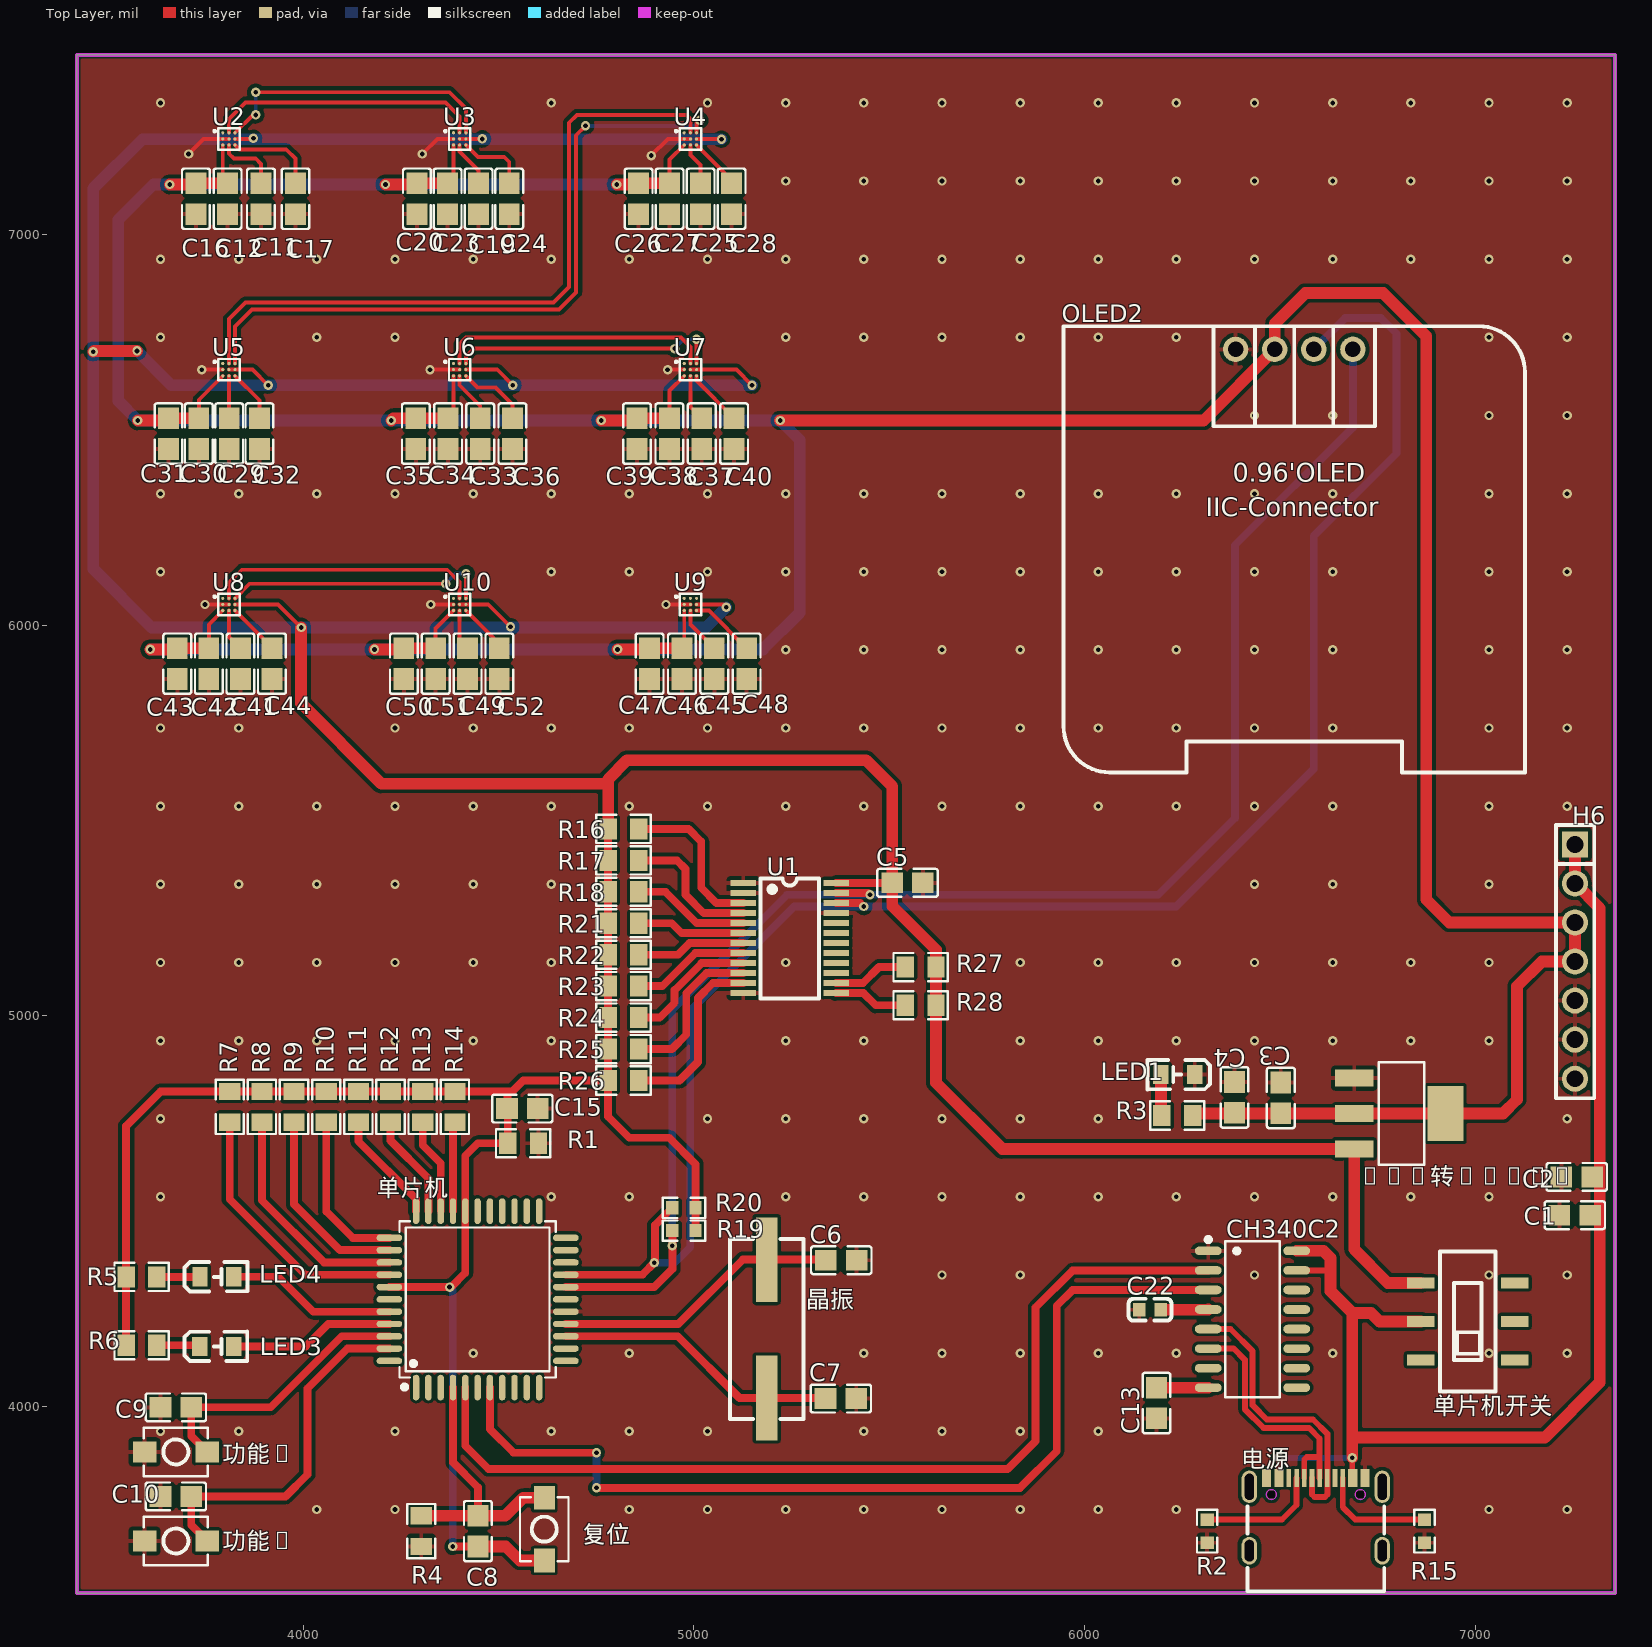
[diagram p0: Top Layer view]
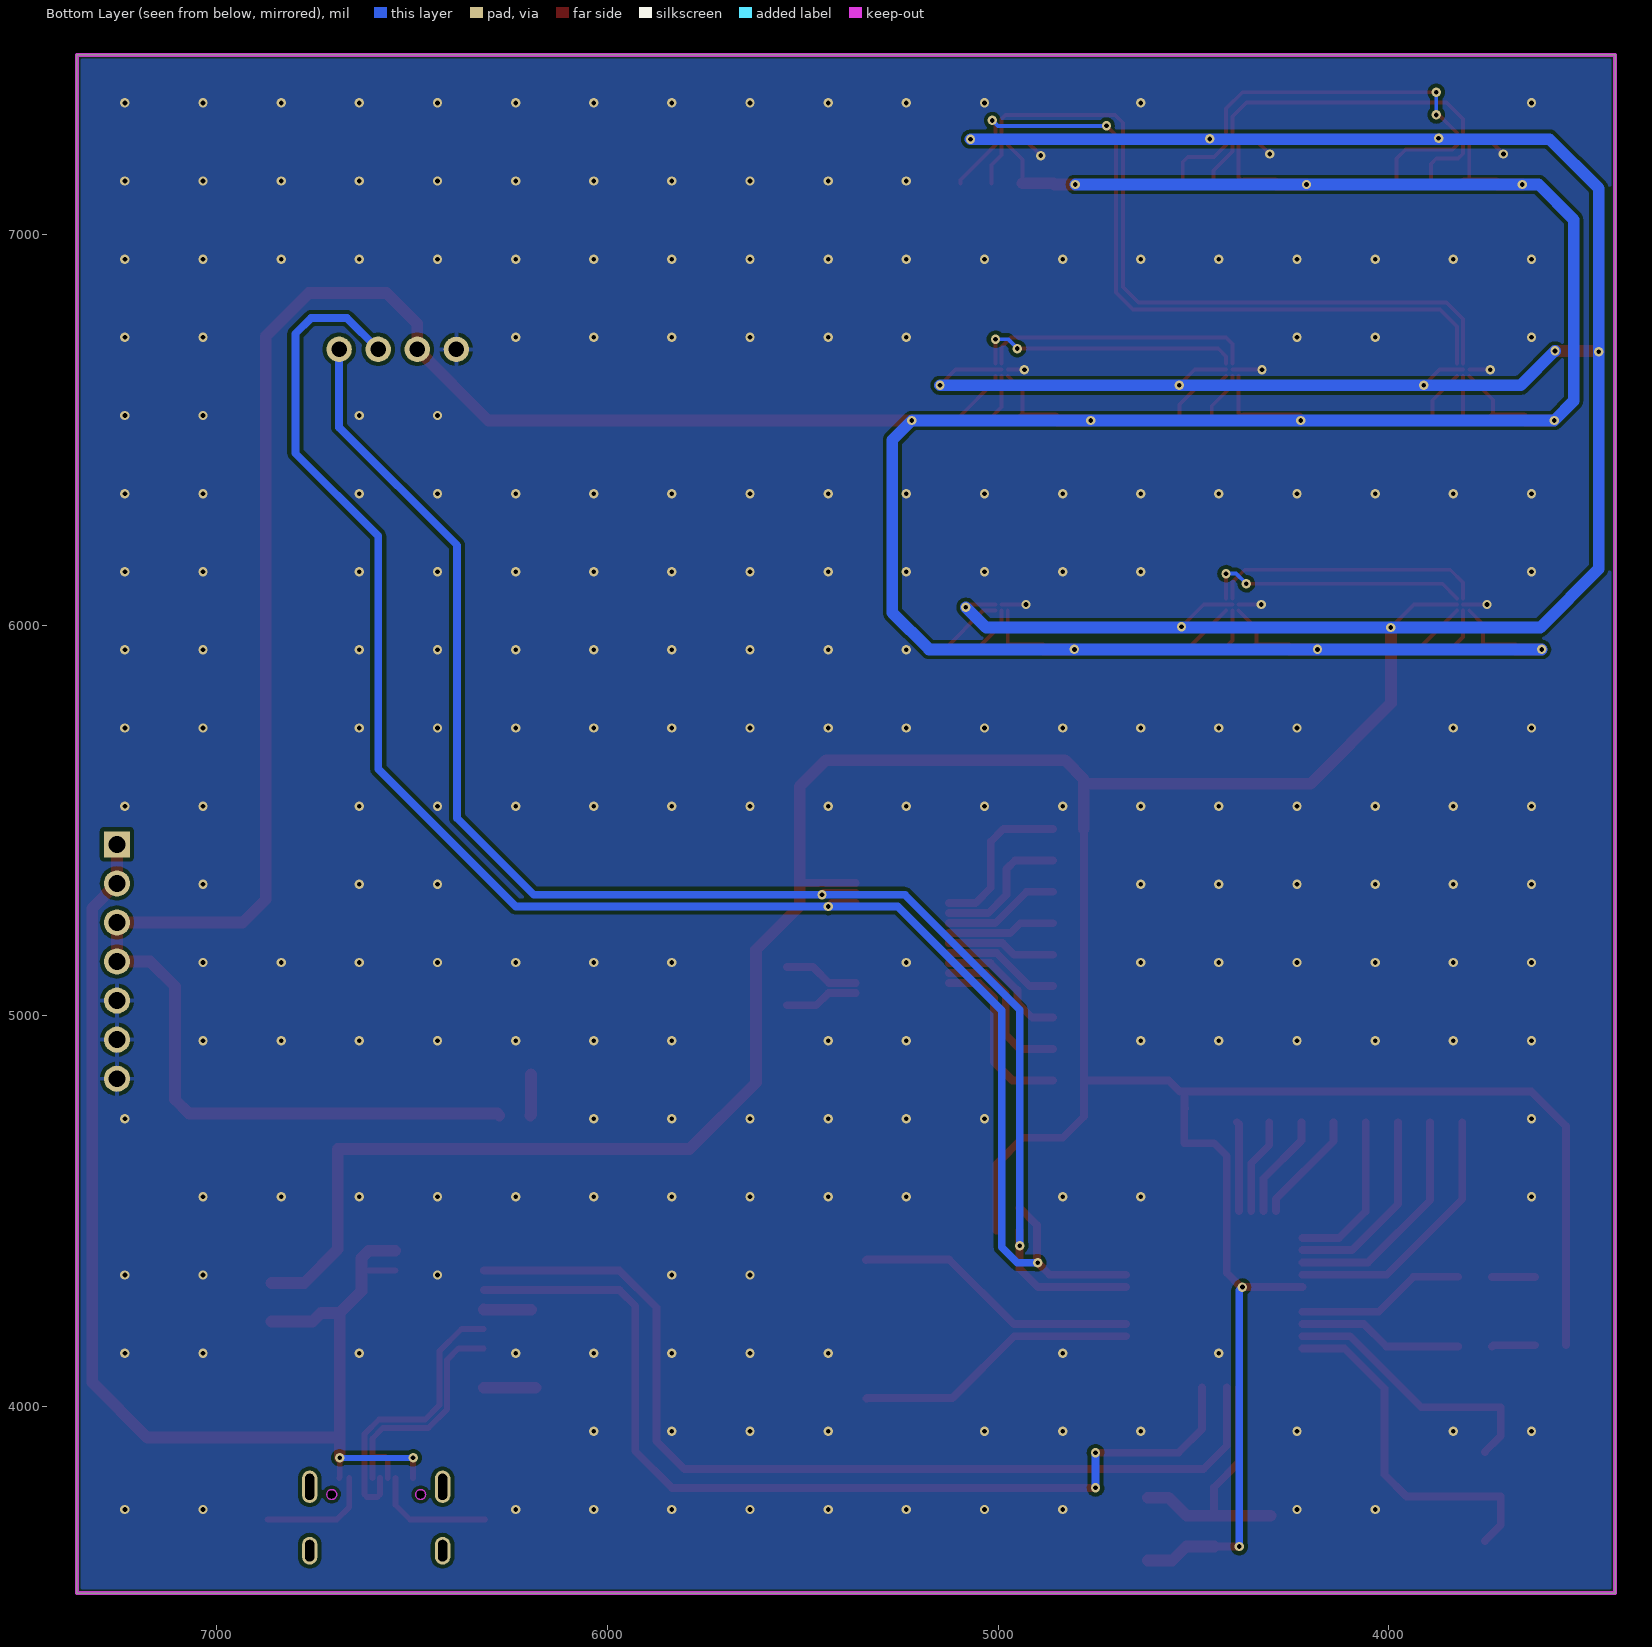
[diagram p1: Bottom Layer view, seen from below]
# Altium PCB MISC75115.pcbdoc
Units mil, origin at the board's own origin, x right, y up, seen from the top; angles counter-clockwise.
Board outline 3937.01 x 3937.01 mil, 2 copper layers (Top Layer, Bottom Layer), stack 62.206 mil thick; 101 components, 93 nets, 370 pads, 280 vias.

## Layer stack, top to bottom
Top Solder Mask Layer: solder mask 0.394, Dk 3.3
Top Layer: signal copper 1.379
Dielectric1: surface 59.449, FR4, Dk 4.5
Bottom Layer: signal copper 1.378
Bottom Solder Mask Layer: solder mask 0.394, Dk 3.3

## Board outline
3420.99,7459.65 3420.99,3522.65 7358,3522.65 7358,7459.65

## Design rules (kind name [scope] priority, off if disabled: settings)
BoardOutlineClearance copperThickness2oz_1 [All] p2 off: genericclearance=7.99 ignorepadtopadclearanceinfootprint=FALSE except(0: Arc-SplitContinuation Track-SplitContinuation SMDPad-SplitContinuation THPad-SplitContinuation Via-SplitContinuation Fill-SplitContinuation Region-SplitContinuation Poly-SplitContinuation Text-SplitContinuation Hole-SplitContinuation; 5.98: Arc-CutoutEdge SMDPad-CutoutEdge THPad-CutoutEdge Via-CutoutEdge Fill-CutoutEdge Region-CutoutEdge Text-CutoutEdge; 6.93: Hole-OutlineEdge Hole-CutoutEdge; 10: Poly-OutlineEdge Poly-CutoutEdge; 11.81: Arc-OutlineEdge Track-OutlineEdge SMDPad-OutlineEdge THPad-OutlineEdge Via-OutlineEdge Fill-OutlineEdge Region-OutlineEdge Text-OutlineEdge Track-CutoutEdge)
BoardOutlineClearance Plane_innerPlane_1 [All] p4 off: genericclearance=4.02 ignorepadtopadclearanceinfootprint=FALSE except(0: Arc-SplitContinuation Track-SplitContinuation SMDPad-SplitContinuation THPad-SplitContinuation Via-SplitContinuation Fill-SplitContinuation Region-SplitContinuation Poly-SplitContinuation Text-SplitContinuation Hole-SplitContinuation; 6: SMDPad-CutoutEdge THPad-CutoutEdge Via-CutoutEdge Fill-CutoutEdge Region-CutoutEdge Text-CutoutEdge; 6.93: Hole-OutlineEdge Hole-CutoutEdge; 10: Poly-OutlineEdge Poly-CutoutEdge; 11.8: Arc-OutlineEdge Track-OutlineEdge SMDPad-OutlineEdge THPad-OutlineEdge Via-OutlineEdge Fill-OutlineEdge Region-OutlineEdge Text-OutlineEdge; 11.81: Arc-CutoutEdge Track-CutoutEdge)
BoardOutlineClearance Copper_copperRegion_1 [All] p6 off: genericclearance=4.02 ignorepadtopadclearanceinfootprint=FALSE except(0: Arc-SplitContinuation Track-SplitContinuation SMDPad-SplitContinuation THPad-SplitContinuation Via-SplitContinuation Fill-SplitContinuation Region-SplitContinuation Poly-SplitContinuation Text-SplitContinuation Hole-SplitContinuation; 6: SMDPad-CutoutEdge THPad-CutoutEdge Via-CutoutEdge Fill-CutoutEdge Region-CutoutEdge Text-CutoutEdge; 6.93: Hole-OutlineEdge Hole-CutoutEdge; 10: Poly-OutlineEdge Poly-CutoutEdge; 11.8: Arc-OutlineEdge Track-OutlineEdge SMDPad-OutlineEdge THPad-OutlineEdge Via-OutlineEdge Fill-OutlineEdge Region-OutlineEdge Text-OutlineEdge; 11.81: Arc-CutoutEdge Track-CutoutEdge)
BoardOutlineClearance copperThickness1oz_1 [All] p8: genericclearance=4.02 ignorepadtopadclearanceinfootprint=FALSE except(0: Arc-SplitContinuation Track-SplitContinuation SMDPad-SplitContinuation THPad-SplitContinuation Via-SplitContinuation Fill-SplitContinuation Region-SplitContinuation Poly-SplitContinuation Text-SplitContinuation Hole-SplitContinuation; 6: SMDPad-CutoutEdge THPad-CutoutEdge Via-CutoutEdge Fill-CutoutEdge Region-CutoutEdge Text-CutoutEdge; 6.93: Hole-OutlineEdge Hole-CutoutEdge; 10: Poly-OutlineEdge Poly-CutoutEdge; 11.8: Arc-OutlineEdge Track-OutlineEdge SMDPad-OutlineEdge THPad-OutlineEdge Via-OutlineEdge Fill-OutlineEdge Region-OutlineEdge Text-OutlineEdge; 11.81: Arc-CutoutEdge Track-CutoutEdge)
Clearance copperThickness2oz [All] p1 off: gap=7.99 ignorepadtopadclearanceinfootprint=FALSE except(5.98: SMDPad-Track SMDPad-SMDPad THPad-Track SMDPad-THPad THPad-THPad Track-Via SMDPad-Via THPad-Via Via-Via Fill-Track Region-Track Fill-SMDPad Region-SMDPad Fill-THPad Region-THPad Fill-Via Region-Via Fill-Fill Fill-Region Region-Region Arc-Track Arc-SMDPad Arc-THPad Arc-Via Fill-Arc Region-Arc Arc-Arc Text-Track SMDPad-Text Text-THPad Text-Via Fill-Text Region-Text Arc-Text Text-Text; 6.93: Hole-Track Hole-SMDPad Hole-THPad Hole-Via Fill-Hole Region-Hole Hole-Arc Hole-Text; 10: Poly-Track Poly-SMDPad Poly-THPad Poly-Via Poly-Fill Poly-Region Poly-Poly Poly-Arc Poly-Text Poly-Hole)
Clearance Plane_innerPlane [All] p3 off: gap=4.02 ignorepadtopadclearanceinfootprint=FALSE except(4.33: SMDPad-Track SMDPad-SMDPad SMDPad-THPad; 5.98: THPad-Track THPad-THPad Track-Via SMDPad-Via THPad-Via Via-Via Fill-Track Region-Track Fill-SMDPad Region-SMDPad Fill-THPad Region-THPad Fill-Via Region-Via Fill-Fill Fill-Region Region-Region; 6: Arc-Track Arc-SMDPad Arc-THPad Arc-Via Fill-Arc Region-Arc Arc-Arc Text-Track SMDPad-Text Text-THPad Text-Via Fill-Text Region-Text Arc-Text Text-Text; 6.93: Hole-Track Hole-SMDPad Hole-THPad Hole-Via Fill-Hole Region-Hole Hole-Arc Hole-Text; 10: Poly-Track Poly-SMDPad Poly-THPad Poly-Via Poly-Fill Poly-Region Poly-Poly Poly-Arc Poly-Text Poly-Hole)
Clearance Copper_copperRegion [All] p5 off: gap=4.02 ignorepadtopadclearanceinfootprint=FALSE except(4.33: SMDPad-Track SMDPad-SMDPad SMDPad-THPad; 5.98: THPad-Track THPad-THPad Track-Via SMDPad-Via THPad-Via Via-Via Fill-Track Region-Track Fill-SMDPad Region-SMDPad Fill-THPad Region-THPad Fill-Via Region-Via Fill-Fill Fill-Region Region-Region; 6: Arc-Track Arc-SMDPad Arc-THPad Arc-Via Fill-Arc Region-Arc Arc-Arc Text-Track SMDPad-Text Text-THPad Text-Via Fill-Text Region-Text Arc-Text Text-Text; 6.93: Hole-Track Hole-SMDPad Hole-THPad Hole-Via Fill-Hole Region-Hole Hole-Arc Hole-Text; 10: Poly-Track Poly-SMDPad Poly-THPad Poly-Via Poly-Fill Poly-Region Poly-Poly Poly-Arc Poly-Text Poly-Hole)
Clearance copperThickness1oz [All] p7: gap=4.02 ignorepadtopadclearanceinfootprint=FALSE except(4.33: SMDPad-Track SMDPad-SMDPad SMDPad-THPad; 5.98: THPad-Track THPad-THPad Track-Via SMDPad-Via THPad-Via Via-Via Fill-Track Region-Track Fill-SMDPad Region-SMDPad Fill-THPad Region-THPad Fill-Via Region-Via Fill-Fill Fill-Region Region-Region; 6: Arc-Track Arc-SMDPad Arc-THPad Arc-Via Fill-Arc Region-Arc Arc-Arc Text-Track SMDPad-Text Text-THPad Text-Via Fill-Text Region-Text Arc-Text Text-Text; 6.93: Hole-Track Hole-SMDPad Hole-THPad Hole-Via Fill-Hole Region-Hole Hole-Arc Hole-Text; 7.87: Poly-SMDPad; 10: Poly-Track Poly-THPad Poly-Via Poly-Fill Poly-Region Poly-Poly Poly-Arc Poly-Text Poly-Hole)
DiffPairsRouting differentialPair [All] p1: maxlimit=6 minlimit=6 mostfreqgap=6 toplayer_minwidth=5 toplayer_prefwidth=10 toplayer_maxwidth=100 toplayer_mingap=6 toplayer_prefgap=6 toplayer_maxgap=6 bottomlayer_minwidth=5 bottomlayer_prefwidth=10 bottomlayer_maxwidth=100 bottomlayer_mingap=6 bottomlayer_prefgap=6 bottomlayer_maxgap=6 maxuncoupledlength=10
HoleToHoleClearance otherClearance [All] p1: gap=11.81 allowstackedmicrovias=TRUE
Length netLength [All] p1: minlimit=0 maxlimit=0
MatchedLengths netLengthTolerance [All] p1: tolerance=1000
PasteMaskExpansion pasteMaskExpansion [All] p1: expansion=0
PlaneConnect innerPlane [All] p1: planeconnectstyle=Relief reliefexpansion=20 reliefentries=4 reliefconductorwidth=10 reliefairgap=10
PolygonConnect copperRegion [(InNet('GND'))] p1: connectstyle=Relief reliefconductorwidth=10 reliefentries=4 polygonreliefangle="90 Angle" airgapwidth=10 via.connectstyle=Relief via.reliefconductorwidth=10 via.reliefentries=4 via.polygonreliefangle="90 Angle" via.airgapwidth=10
RoutingVias viaSize [All] p1: holewidth=12.01 width=24.02 viastyle="Through Hole" minholewidth=11.81 minwidth=19.68 maxholewidth=248.03 maxwidth=393.7
SolderMaskExpansion solderMaskExpansion [IsVia] p1: expansion=-1000 istentingtop=TRUE
SolderMaskExpansion solderMaskExpansion [All] p2: expansion=2 istentingtop=FALSE
Width copperThickness2oz_2 [All] p1 off: maxlimit=100 minlimit=8 preferedwidth=10
Width copperThickness1oz_2 [All] p2: maxlimit=100 minlimit=5 preferedwidth=10

## Components (designator, comment, footprint, x,y, rotation, side; value= is the part's Value field where it differs from the comment)
+5v转+3.3v "AMS1117-3.3" SOT-223-3_L6.5-W3.4-P2.30-LS7.0-BR 6807.33,4750.06 r180 top (schematic designator +5vת+3.3v)
C1 "10UF" C0805 7254.78,4489.81 r0 top
C2 "100nF" C0805 7259.73,4587.87 r0 top
C3 "100nF" C0805 6502.33,4790.06 r270 top
C4 "10UF" C0805 6383.84,4791.38 r270 top
C5 "100nF" C0805 5546.9,5340.64 r0 top
C6 "22PF" C0805 5377.38,4374.53 r0 top
C7 "22PF" C0805 5376.25,4020.68 r0 top
C8 "10UF" C0805 4447.29,3681.27 r90 top
C9 "0.1uf" C0805 3674.24,3998.11 r0 top
C10 "0.1uf" C0805 3674.24,3770.08 r0 top
C11 "2.2uF" C0805 3892.09,7091.39 r270 top
C12 "10UF" C0805 3806.59,7091.39 r270 top
C13 "0.1UF" C0805 6184.26,4009.17 r90 top
C15 "0.1uF" C0805 4561.03,4762.76 r180 top
C16 "0.1UF" C0805 3725.76,7091.39 r90 top
C17 "0.1UF" C0805 3980.5,7091.39 r90 top
C19 "2.2uF" C0805 4449.23,7091.39 r270 top
C20 "10UF" C0805 4291.41,7091.39 r270 top
C22 "100nF" C0603 6167.65,4248 r0 top
C23 "0.1UF" C0805 4369.72,7091.39 r90 top
C24 "0.1UF" C0805 4527.68,7091.39 r90 top
C25 "2.2uF" C0805 5017.41,7091.39 r270 top
C26 "10UF" C0805 4858.71,7091.39 r270 top
C27 "0.1UF" C0805 4938.06,7091.39 r90 top
C28 "0.1UF" C0805 5096.75,7091.39 r90 top
C29 "2.2uF" C0805 3810.7,6490.3 r270 top
C30 "10UF" C0805 3733.09,6490.3 r270 top
C31 "0.1UF" C0805 3655.48,6490.3 r90 top
C32 "0.1UF" C0805 3888.3,6490.3 r90 top
C33 "2.2uF" C0805 4453.38,6490.3 r270 top
C34 "10UF" C0805 4370.98,6490.3 r270 top
C35 "0.1UF" C0805 4288.57,6490.3 r90 top
C36 "0.1UF" C0805 4535.78,6490.3 r90 top
C37 "2.2uF" C0805 5020.24,6490.3 r270 top
C38 "10UF" C0805 4937.42,6490.3 r270 top
C39 "0.1UF" C0805 4854.6,6490.3 r90 top
C40 "0.1UF" C0805 5103.06,6490.3 r90 top
C41 "2.2uF" C0805 3839.49,5901.41 r270 top
C42 "10UF" C0805 3758.74,5901.41 r270 top
C43 "0.1UF" C0805 3677.99,5901.41 r90 top
C44 "0.1UF" C0805 3920.25,5901.41 r90 top
C45 "2.2uF" C0805 5052.43,5901.41 r270 top
C46 "10UF" C0805 4969.58,5901.41 r270 top
C47 "0.1UF" C0805 4886.73,5901.41 r90 top
C48 "0.1UF" C0805 5135.28,5901.41 r90 top
C49 "2.2uF" C0805 4420.81,5901.41 r270 top
C50 "10UF" C0805 4257.85,5901.41 r270 top
C51 "0.1UF" C0805 4339.33,5901.41 r90 top
C52 "0.1UF" C0805 4502.28,5901.41 r90 top
CH340C2 "CH340C" SOP-16_L10.0-W3.9-P1.27-LS6.0-BL 6429.8,4223.56 r270 top
H6 "" HDR-TH_7P-P2.54-V-M 7255.44,5139.1 r270 top
LED1 "" LED_0805 6236.85,4849.96 r180 top
LED3 "" LED_0805 3781.01,4153.88 r0 top
LED4 "" LED_0805 3781.45,4331.99 r0 top
OLED2 "0.96OLED_4P_MODULE_JX" 0.96OLED_4P 6536.78,6705.99 r0 top
R1 "1K" R0805 4563.04,4674.02 r180 top
R2 "5.1K" R0603 6313.91,3681.25 r90 top
R3 "1K" R0805 6237.33,4745.06 r180 top
R4 "10K" R0805 4302.29,3681.27 r90 top
R5 "1K" R0805 3586.45,4331.99 r180 top
R6 "1K" R0805 3586.45,4156.99 r180 top
R7 "10K" R0805 3812.09,4767.13 r90 top
R8 "10K" R0805 3894.42,4767.13 r90 top
R9 "10K" R0805 3976.74,4767.13 r90 top
R10 "10K" R0805 4059.06,4767.13 r90 top
R11 "10K" R0805 4141.39,4767.13 r90 top
R12 "10K" R0805 4223.71,4767.13 r90 top
R13 "10K" R0805 4306.03,4767.13 r90 top
R14 "10K" R0805 4388.35,4767.13 r90 top
R15 "5.1K" R0603 6870.09,3681.25 r90 top
R16 "10K" R0805 4820.05,5478.59 r0 top
R17 "4.7K" R0805 4820.05,5398.1 r0 top
R18 "4.7K" R0805 4820.05,5317.6 r0 top
R19 "4.7K" R0603 4974.74,4450.48 r180 top
R20 "4.7K" R0603 4974.74,4508.71 r180 top
R21 "4.7K" R0805 4820.05,5237.11 r0 top
R22 "4.7K" R0805 4820.05,5156.62 r0 top
R23 "4.7K" R0805 4820.05,5076.13 r0 top
R24 "4.7K" R0805 4820.05,4995.64 r0 top
R25 "4.7K" R0805 4820.05,4915.15 r0 top
R26 "4.7K" R0805 4820.05,4834.65 r0 top
R27 "4.7K" R0805 5580.44,5125 r0 top
R28 "4.7K" R0805 5580.44,5027.11 r0 top
U1 "TCA9548APWR" TSSOP-24_L7.8-W4.4-P0.65-LS6.4-BL 5245.63,5199.05 r270 top
U2 "BMM350" WLCSP-9_L1.3-W1.3-R3-C3-P0.40-TL 3810.08,7244.57 r0 top
U3 "BMM350" WLCSP-9_L1.3-W1.3-R3-C3-P0.40-TL 4400.64,7244.57 r0 top
U4 "BMM350" WLCSP-9_L1.3-W1.3-R3-C3-P0.40-TL 4991.21,7244.57 r0 top
U5 "BMM350" WLCSP-9_L1.3-W1.3-R3-C3-P0.40-TL 3810.08,6654.02 r0 top
U6 "BMM350" WLCSP-9_L1.3-W1.3-R3-C3-P0.40-TL 4400.64,6654.02 r0 top
U7 "BMM350" WLCSP-9_L1.3-W1.3-R3-C3-P0.40-TL 4991.21,6654.02 r0 top
U8 "BMM350" WLCSP-9_L1.3-W1.3-R3-C3-P0.40-TL 3810.08,6053.06 r0 top
U9 "BMM350" WLCSP-9_L1.3-W1.3-R3-C3-P0.40-TL 4991.21,6053.06 r0 top
U10 "BMM350" WLCSP-9_L1.3-W1.3-R3-C3-P0.40-TL 4400.64,6053.06 r0 top
功能1 "Tact switch 3*4*H" SW-SMD_L4.0-W2.9-LS5.0 3674.24,3884.1 r180 top
功能2 "Tact switch 3*4*H" SW-SMD_L4.0-W2.9-LS5.0 3674.24,3656.07 r180 top
单片机 "STC89C52RC-40I-LQFP44" LQFP-44_L10.0-W10.0-P0.80-LS12.0-BL 4446.58,4274.46 r0 top
单片机开关 "SS-3235S-L1" SW-SMD_SS-3235S-LX 6980.85,4217.96 r270 top
复位 "Tact switch 3*4*H" SW-SMD_L4.0-W2.9-LS5.0 4617.29,3686.27 r270 top
晶振 "12MHz" CRYSTAL-SMD_L11.4-W4.7-LS12.7 5186.58,4199.09 r270 top
电源 "Type-C" USB-C-SMD_TYPE-C16PIN 6592,3724.3 r0 top

## Footprints (in the part's own frame and the unit in brackets; to place one, negate y for a bottom-side part, rotate by r counter-clockwise, add the part's x,y. Pads: shape width x height; smd on the part's side, far side on the other; paste and mask are expansions set on the pad)
0.96OLED_4P [mm]
  round 1.65 hole 1 copper offset 0,0: 1(-3.81,-0.001) 2(-1.27,0.002) 3(1.27,0.002) 4(3.81,0.002)
  silkscreen extent -15,-27.5 15,1.5
C0603 [mm]
  rect 0.8x0.9 smd: 1(-0.7,0) 2(0.7,0)
  silkscreen extent -1.39,-0.71 1.39,0.71
C0805 [mm]
  rect 1.41x1.35 smd paste-100 mask+0.051: 1(-1,0) 2(1,0)
  silkscreen extent -1.96,-0.9 1.96,0.9
CRYSTAL-SMD_L11.4-W4.7-LS12.7 [mm]
  rect 5.5x1.4 smd: 1(-4.5,0) 2(4.5,0)
  silkscreen extent -5.85,-2.4 5.85,2.4
HDR-TH_7P-P2.54-V-M [mm]
  rect 1.7x1.7 hole 1.1: 1(-7.62,0)
  round 1.7 hole 1.1: 2(-5.08,0) 3(-2.54,0) 4(0,0) 5(2.54,0) 6(5.08,0) 7(7.62,0)
  silkscreen extent -8.89,-1.25 8.89,1.25
LED_0805 [mm]
  rect 1x1.25 smd paste+0 mask+0.051: 1(-1.15,0.005) 2(1.05,0.005)
  silkscreen extent -2.15,-0.94 1.93,0.97
LQFP-44_L10.0-W10.0-P0.80-LS12.0-BL [mm]
  oval 0.42x1.67 smd: 1(-4,-5.735) 2(-3.2,-5.735) 3(-2.4,-5.735) 4(-1.6,-5.735) 5(-0.8,-5.735) 6(0,-5.735) 7(0.8,-5.735) 8(1.6,-5.735) 9(2.4,-5.735) 10(3.2,-5.735) 11(4,-5.735) 23(4,5.735) 24(3.2,5.735) 25(2.4,5.735) 26(1.6,5.735) 27(0.8,5.735) 28(0,5.735) 29(-0.8,5.735) 30(-1.6,5.735) 31(-2.4,5.735) 32(-3.2,5.735) 33(-4,5.735)
  oval 1.67x0.42 smd: 12(5.735,-4) 13(5.735,-3.2) 14(5.735,-2.4) 15(5.735,-1.6) 16(5.735,-0.8) 17(5.735,0) 18(5.735,0.8) 19(5.735,1.6) 20(5.735,2.4) 21(5.735,3.2) 22(5.735,4) 34(-5.735,4) 35(-5.735,3.2) 36(-5.735,2.4) 37(-5.735,1.6) 38(-5.735,0.8) 39(-5.735,0) 40(-5.735,-0.8) 41(-5.735,-1.6) 42(-5.735,-2.4) 43(-5.735,-3.2) 44(-5.735,-4)
  silkscreen extent -5.08,-5.85 5.08,5.08
R0603 [mil]
  rect 31.75x34.02 smd paste-3937.01 mask+2: 1(-29.66,0) 2(29.66,0)
  silkscreen extent -55,-26 55,26
R0805 [mm]
  rect 1.133x1.377 smd paste-100 mask+0.051: 1(-1,0) 2(1,0)
  silkscreen extent -1.76,-0.92 1.76,0.92
SOP-16_L10.0-W3.9-P1.27-LS6.0-BL [mm]
  oval 0.56x1.745 smd: 1(-4.445,-2.872) 2(-3.175,-2.872) 3(-1.905,-2.872) 4(-0.635,-2.872) 5(0.635,-2.872) 6(1.905,-2.872) 7(3.175,-2.872) 8(4.445,-2.872) 9(4.445,2.872) 10(3.175,2.872) 11(1.905,2.872) 12(0.635,2.872) 13(-0.635,2.872) 14(-1.905,2.872) 15(-3.175,2.872) 16(-4.445,2.872)
  silkscreen extent -5.33,-3.02 5.08,1.77
SOT-223-3_L6.5-W3.4-P2.30-LS7.0-BR [mm]
  rect 2.5x1.1 smd: 1(2.97,-2.3) 2(2.97,0) 3(2.97,2.3)
  rect 2.34x3.6 smd: 4(-2.97,0)
  silkscreen extent -1.57,-3.33 1.37,3.33
SW-SMD_L4.0-W2.9-LS5.0 [mm]
  rect 1.53x1.36 smd: 1(-2.035,0) 2(2.035,0)
  silkscreen extent -2.08,-1.58 2.08,1.58
SW-SMD_SS-3235S-LX [mm]
  rect 0.7x1.8 smd: 1(-2.5,3.05) 2(0,3.05) 3(2.5,3.05) 4(-2.5,-3.05) 5(0,-3.05) 6(2.5,-3.05)
  silkscreen extent -4.55,-1.8 4.55,1.8
TSSOP-24_L7.8-W4.4-P0.65-LS6.4-BL [mm]
  rect 0.4x1.65 smd: 1(-3.575,-3.023) 2(-2.925,-3.023) 3(-2.275,-3.023) 4(-1.625,-3.023) 5(-0.975,-3.023) 6(-0.325,-3.023) 7(0.325,-3.023) 8(0.975,-3.023) 9(1.625,-3.023) 10(2.275,-3.023) 11(2.925,-3.023) 12(3.575,-3.023) 13(3.575,3.023) 14(2.925,3.023) 15(2.275,3.023) 16(1.625,3.023) 17(0.975,3.023) 18(0.325,3.023) 19(-0.325,3.023) 20(-0.975,3.023) 21(-1.625,3.023) 22(-2.275,3.023) 23(-2.925,3.023) 24(-3.575,3.023)
  silkscreen extent -3.89,-1.91 3.94,1.91
USB-C-SMD_TYPE-C16PIN [mm]
  oval 1x2.1 hole 0.6 slot 1.7 at 90 deg: 1(-4.32,1.787) 2(4.32,1.787)
  oval 1x1.8 hole 0.6 slot 1.4 at 90 deg: 3(-4.32,-2.362) 4(4.32,-2.362)
  rect 0.6x1.15 smd paste-100 mask+0.051: A1B12(-3.2,2.362) A4B9(-2.4,2.362) B1A12(3.2,2.362) B4A9(2.4,2.362)
  rect 0.3x1.15 smd paste-100 mask+0.051: A5(-1.25,2.362) A6(-0.25,2.362) A7(0.25,2.362) A8(1.25,2.362) B5(1.75,2.362) B6(0.75,2.362) B7(-0.75,2.362) B8(-1.75,2.362)
  Board Outline Layer circle w0.003: c2.89,1.288 r0.325
  Board Outline Layer circle w0.003: c-2.89,1.288 r0.325
  Board Outline Layer region: 3.215,1.288 3.183,1.147 3.093,1.034 2.962,0.971 2.818,0.971 2.687,1.034 2.597,1.147 2.565,1.288 2.565,1.288 2.597,1.429 2.687,1.542 2.818,1.605 2.962,1.605 3.093,1.542 3.183,1.429 3.215,1.288
  Board Outline Layer region: 3.215,1.288 3.206,1.21 3.178,1.137 3.133,1.073 3.075,1.021 3.005,0.984 2.929,0.965 2.851,0.965 2.775,0.984 2.705,1.021 2.647,1.073 2.602,1.137 2.574,1.21 2.565,1.288 2.574,1.366 2.602,1.439 2.647,1.504 2.705,1.555 2.775,1.592 2.851,1.611 2.929,1.611 3.005,1.592 3.075,1.555 3.133,1.504 3.178,1.439 3.206,1.366
  Board Outline Layer region: -2.565,1.288 -2.597,1.147 -2.687,1.034 -2.818,0.971 -2.962,0.971 -3.093,1.034 -3.183,1.147 -3.215,1.288 -3.215,1.288 -3.183,1.429 -3.093,1.542 -2.962,1.605 -2.818,1.605 -2.687,1.542 -2.597,1.429 -2.565,1.288
  Board Outline Layer region: -2.565,1.288 -2.574,1.21 -2.602,1.137 -2.647,1.073 -2.705,1.021 -2.775,0.984 -2.851,0.965 -2.929,0.965 -3.005,0.984 -3.075,1.021 -3.133,1.073 -3.178,1.137 -3.206,1.21 -3.215,1.288 -3.206,1.366 -3.178,1.439 -3.133,1.504 -3.075,1.555 -3.005,1.592 -2.929,1.611 -2.851,1.611 -2.775,1.592 -2.705,1.555 -2.647,1.504 -2.602,1.439 -2.574,1.366
  Multi-Layer board cut-out: 3.215,1.288 3.183,1.147 3.093,1.034 2.962,0.971 2.818,0.971 2.687,1.034 2.597,1.147 2.565,1.288 2.565,1.288 2.597,1.429 2.687,1.542 2.818,1.605 2.962,1.605 3.093,1.542 3.183,1.429 3.215,1.288
  Multi-Layer board cut-out: -2.565,1.288 -2.597,1.147 -2.687,1.034 -2.818,0.971 -2.962,0.971 -3.093,1.034 -3.183,1.147 -3.215,1.288 -3.215,1.288 -3.183,1.429 -3.093,1.542 -2.962,1.605 -2.818,1.605 -2.687,1.542 -2.597,1.429 -2.565,1.288
  silkscreen extent -4.45,-5 4.45,0.52
WLCSP-9_L1.3-W1.3-R3-C3-P0.40-TL [mm]
  round 0.2 smd paste-100 mask+0.051: A1(-0.4,0.4) A2(0,0.4) A3(0.4,0.4) B1(-0.4,0) B2(0,0) B3(0.4,0) C1(-0.4,-0.4) C2(0,-0.4) C3(0.4,-0.4)
  silkscreen extent -1,-0.7 0.7,0.7

## Via types
v1: diameter 24.02, hole 12, Top Layer to Bottom Layer, 280 vias

## Nets (pads, with @x,y where several pads share a name; then routed paths per layer and width w, separated by ;. In a path a pad name is that pad's centre, name@x,y a point inside that pad or via, vN(x,y) a via of type N, cw(c..) or ccw(c..) an arc to the next point about the centre after c; other vN are vias at no path point)
3.3V: +5v转+3.3v.2 +5v转+3.3v.4 C3.2 C4.2 C12.1 C16.2 C20.1 C23.2 C26.1 C27.2 C30.1 C31.2 C34.1 C35.2 C38.1 C39.2 C42.1 C43.2 C46.1 C47.2 C50.1 C51.2 H6.3 H6.4 OLED2.2 R3.1 U2.C1 U3.C1 U4.C1 U5.C1 U6.C1 U7.C1 U8.C1 U9.C1 U10.C1 | length 13260.6
  Top Layer w10: C30.1 3733.09,6577.04 U5.C1 ; C42.1 3758.74,6001.72 U8.C1 ; U2.C1 3794.33,7143.03 C12.1 ; C51.2 4339.33,5991.75 U10.C1 ; C23.2 4384.89,7145.94 U3.C1 ; C34.1 4384.89,6543.58 U6.C1 ; C38.1 4937.42,6600.24 U7.C1 ; C27.2 4938.06,7191.43 U4.C1 ; C46.1 4975.46,5946.66 U9.C1
  Top Layer w30: v1(3576.85,6523.96) 3649.78,6523.96 C31.2 C30.1 ; v1(3608.85,5937.96) 3675.17,5937.96 C43.2 C42.1 ; v1(3658.85,7127.96) 3722.95,7127.96 C16.2 C12.1 ; v1(4182.85,5937.96) 4255.03,5937.96 C50.1 C51.2 ; v1(4210.85,7127.96) 4288.61,7127.96 C20.1 C23.2 ; v1(4225.23,6523.96) 4230.94,6529.67 C35.2 C34.1 ; v1(4762.85,6523.96) 4848.9,6523.96 C39.2 C38.1 ; v1(4802.85,7127.96) 4855.91,7127.96 C26.1 C27.2 ; v1(4804.85,5937.96) 4883.9,5937.96 C47.2 C46.1 ; v1(5220.85,6523.96) 6304.7,6523.96 6486.78,6706.04 6486.78,6771.89 6564.85,6849.96 6764.85,6849.96 6874.85,6739.96 6874.85,5297.9 6933.65,5239.1 H6.3 H6.4 7169.99,5139.1 7106.85,5075.96 7106.85,4785.96 7070.95,4750.06 +5v转+3.3v.4 +5v转+3.3v.2 6281.7,4750.06 R3.1
  Bottom Layer w30: v1(3608.85,5937.96) v1(4182.85,5937.96) v1(4804.85,5937.96) 5176.85,5937.96 5270.85,6031.96 5270.85,6473.96 v1(5220.85,6523.96) v1(4762.85,6523.96) v1(4225.23,6523.96) v1(3576.85,6523.96) 3526.85,6573.96 3526.85,7037.96 3616.85,7127.96 v1(3658.85,7127.96) v1(4210.85,7127.96) v1(4802.85,7127.96)
$1N1944: LED4.1 R5.1 | length 110.4
  Top Layer w20: R5.1 3735.97,4331.99 LED4.1
$1N1945: LED3.1 R6.1 | length 111.1
  Top Layer w20: R6.1 3732.83,4156.99 LED3.1
$1N2954: LED1.2 R3.2 | length 105.7
  Top Layer w30: LED1.2 6195.51,4747.52 R3.2
$1N3992: C22.2 CH340C2.4 | length 121.7
  Top Layer w30: C22.2 6316.15,4248 CH340C2.4
$1N3994: R15.2 电源.B5 | length 296.9
  Top Layer w15: 电源.B5 6660.9,3742.74 6692.73,3710.91 R15.2
$1N3995: R2.2 电源.A5 | length 313.3
  Top Layer w15: R2.2 6505.32,3710.91 6542.79,3748.38 电源.A5
$1N4005: CH340C2.6 电源.A7 电源.B7 | length 647.2
  Top Layer w15: CH340C2.6 6381.57,4148.56 6410.28,4119.85 6410.28,3993.35 6458.47,3945.17 6574.93,3945.17 6601.6,3918.5 6601.6,3864.28 ; 电源.B7 6562.47,3864.43 6568.91,3870.87 6595.01,3870.87 6601.6,3864.28 ; 电源.A7 6601.6,3817.55 6601.6,3864.28
$1N4006: CH340C2.5 电源.A6 电源.B6 | length 739.6
  Top Layer w15: CH340C2.5 6373.74,4198.56 6430.36,4141.94 6430.36,4003.39 6466.5,3967.25 6584.97,3967.25 6621.53,3930.69 电源.B6 6621.53,3774.91 6615.09,3768.47 6588.98,3768.47 6582.16,3775.3 电源.A6
$1N4007: C13.2 CH340C2.8 | length 132.4
  Top Layer w30: C13.2@6184.28,4048.56 CH340C2.8
$1N4040: C1.2 C2.2 CH340C2.15 CH340C2.16 H6.1 H6.2 单片机开关.5 电源.A4B9 电源.B4A9 | length 3287
  Top Layer w15: 电源.A4B9 v1(6497.51,3868.87) ; CH340C2.15 6629.8,4348.56 ; v1(6685.36,3868.87) 6685.36,3818.43 电源.B4A9
  Top Layer w30: CH340C2.16 6611.45,4398.56 6629.8,4380.21 6629.8,4348.56 6629.8,4295.38 6685.36,4239.82 ; v1(6685.36,3868.87) 6685.36,3920.83 ; 单片机开关.5 6754.86,4217.96 6732.99,4239.82 6685.36,4239.82 ; H6.1 H6.2 7318.85,5275.69 7318.85,4061.96 7177.72,3920.83 6685.36,3920.83 ; 6685.36,3920.83 6685.36,4239.82
  Bottom Layer w15: v1(6497.51,3868.87) v1(6685.36,3868.87)
$2N8: C11.1 U2.C2 | length 164.8
  Top Layer w10: U2.C2 3810.08,7206.74 3822.85,7193.96 3878.85,7193.96 3892.09,7180.72 C11.1
$2N9: C17.2 U2.C3 | length 232.5
  Top Layer w10: U2.C3 3836.69,7217.96 3956.85,7217.96 3980.5,7194.31 C17.2
$2N18: C19.1 U3.C2 | length 118.2
  Top Layer w10: U3.C2 4400.64,7212.17 4449.23,7163.58 C19.1
$2N19: C24.2 U3.C3 | length 183.8
  Top Layer w10: U3.C3 4447.26,7197.96 4514.85,7197.96 4527.68,7185.13 C24.2
$2N28: C25.1 U4.C2 | length 108.9
  Top Layer w10: U4.C2 4991.21,7203.6 5017.41,7177.41 C25.1
$2N29: C28.2 U4.C3 | length 135.3
  Top Layer w10: U4.C3 5096.75,7139.03 C28.2
$2N38: C29.1 U5.C2 | length 108.9
  Top Layer w10: U5.C2 3810.08,6530.29 C29.1
$2N39: C32.2 U5.C3 | length 134.5
  Top Layer w10: U5.C3 3888.3,6575.8 C32.2
$2N48: C33.1 U6.C2 | length 130.5
  Top Layer w10: U6.C2 4400.64,6614.17 4453.38,6561.43 C33.1
$2N49: C36.2 U6.C3 | length 185.1
  Top Layer w10: U6.C3 4446.7,6607.96 4492.85,6607.96 4535.78,6565.03 C36.2
$2N58: C37.1 U7.C2 | length 120.6
  Top Layer w10: U7.C2 4991.21,6558.7 C37.1
$2N59: C40.2 U7.C3 | length 148.4
  Top Layer w10: U7.C3 5006.96,6625.77 C40.2
$2N68: C41.1 U8.C2 | length 108.7
  Top Layer w10: U8.C2 3810.08,5970.2 C41.1
$2N69: C44.2 U8.C3 | length 135.6
  Top Layer w10: U8.C3 3920.25,5942.89 C44.2
$2N78: C45.1 U9.C2 | length 121.9
  Top Layer w10: U9.C2 4991.21,6002.01 C45.1
$2N79: C48.2 U9.C3 | length 168.3
  Top Layer w10: U9.C3 5038.76,6037.31 C48.2
$2N88: C49.1 U10.C2 | length 104.9
  Top Layer w10: U10.C2 4400.64,5960.95 C49.1
$2N89: C52.2 U10.C3 | length 132.1
  Top Layer w10: U10.C3 4502.28,5951.42 C52.2
$2N92: R16.2 U1.3 | length 415
  Top Layer w20: R16.2 4986.22,5478.59 5018.85,5445.96 5018.85,5327.96 5058.2,5288.61 U1.3
$2N103: R17.2 U1.4 | length 361.8
  Top Layer w20: R17.2 4956.71,5398.1 4978.85,5375.96 4978.85,5309.96 5025.79,5263.02 U1.4
$2N104: R18.2 U1.5 | length 300.4
  Top Layer w20: R18.2 4927.21,5317.6 5007.38,5237.43 U1.5
$2N105: R21.2 U1.6 | length 277.7
  Top Layer w20: R21.2 4943.7,5237.11 4968.97,5211.84 U1.6
$2N106: R22.2 U1.7 | length 279.5
  Top Layer w20: R22.2 4959.51,5156.62 4989.15,5186.26 U1.7
$2N107: R23.2 U1.8 | length 302.2
  Top Layer w20: R23.2 4919.02,5076.13 5003.55,5160.66 U1.8
$2N108: R24.2 U1.9 | length 343.7
  Top Layer w20: R24.2 4912.53,4995.64 4950.85,5033.96 4950.85,5065.96 5019.96,5135.07 U1.9
$2N109: R25.2 U1.10 | length 409.8
  Top Layer w20: R25.2 4944.04,4915.15 4980.85,4951.96 4980.85,5057.96 5032.37,5109.48 U1.10
$2N110: R26.2 U1.11 | length 466.5
  Top Layer w20: R26.2 4963.54,4834.65 5010.85,4881.96 5010.85,5045.96 5048.78,5083.89 U1.11
$2N111: R27.1 U1.14 | length 193.5
  Top Layer w20: U1.14 5432.78,5083.89 5473.89,5125 R27.1
$2N112: R28.1 U1.13 | length 189.4
  Top Layer w20: U1.13 5434.5,5058.31 5465.71,5027.11 R28.1
"+ 5V_S": +5v转+3.3v.3 C5.1 C8.1 C15.2 R1.2 R5.2 R6.2 R7.2 R8.2 R9.2 R10.2 R11.2 R12.2 R13.2 R14.2 R16.1 R17.1 R18.1 R19.1 R20.1 R21.1 R22.1 R23.1 R24.1 R25.1 R26.1 R27.2 R28.2 U1.24 U2.B3 U3.B2 U3.B3 U4.B3 U5.B2 U5.B3 U6.B3 U7.B2 U7.B3 U8.B3 U9.B3 U10.B2 U10.B3 单片机.29 单片机.38 单片机开关.4 复位.2 | length 16309.5
  Top Layer w10: U5.B2 U5.B3 3870.79,6654.02 v1(3910.85,6613.96) ; U8.B3 3935.75,6053.06 v1(3994.85,5993.96) ; U2.B3 3871.46,7244.57 v1(3872.85,7245.96) ; U10.B2 U10.B3 4473.75,6053.06 v1(4530.85,5995.96) ; U3.B2 U3.B3 v1(4458.85,7244.57) ; U6.B3 4496.79,6654.02 v1(4536.85,6613.96) ; U7.B2 U7.B3 5108.79,6654.02 v1(5148.85,6613.96) ; U9.B3 5075.75,6053.06 v1(5082.85,6045.96) ; U4.B3 5070.24,7244.57 v1(5070.85,7243.96)
  Top Layer w20: R6.2 R5.2 3547.08,4718.19 3635.39,4806.5 R7.2 R8.2 R9.2 R10.2 R11.2 R12.2 R13.2 R14.2 4522.75,4806.5 ; 单片机.38 4378.85,4305.96 4415.08,4342.19 单片机.29 4415.08,4642.19 4446.91,4674.02 R1.2 4523.67,4760.75 C15.2 4522.75,4763.85 4522.75,4806.5 ; v1(4382.85,3641.9) C8.1 ; R16.1 R17.1 R18.1 R21.1 R22.1 R23.1 R24.1 R25.1 R26.1 ; R19.1 R20.1 5004.4,4620.41 4936.85,4687.96 4834.85,4687.96 4780.68,4742.13 R26.1 ; U1.24 5506.68,5339.79 C5.1 ; 4522.75,4806.5 4535.39,4806.5 4563.54,4834.65 R26.1
  Top Layer w30: v1(3462.85,6699.96) 3464.85,6701.96 v1(3574.85,6701.96) ; v1(3994.85,5993.96) 3994.85,5799.96 4200.44,5594.38 4780.68,5594.38 ; C8.1 4518.91,3641.9 4554.66,3606.15 复位.2 ; R16.1 4780.68,5594.38 ; 单片机开关.4 6776.43,4316.39 6690.41,4402.41 +5v转+3.3v.3 5789.3,4659.51 5619.81,4829 R28.2 R27.2 5619.81,5169 5507.53,5281.28 C5.1 5507.53,5587.28 5440.85,5653.96 4828.85,5653.96 4780.68,5605.79 4780.68,5594.38
  Bottom Layer w20: v1(4374.85,4305.96) 4382.85,4297.96 v1(4382.85,3641.9)
  Bottom Layer w30: v1(3574.85,6701.96) 3662.85,6613.96 v1(3910.85,6613.96) v1(4536.85,6613.96) v1(5148.85,6613.96) ; v1(5070.85,7243.96) 3588.85,7243.96 3462.85,7117.96 v1(3462.85,6699.96) 3462.85,6143.96 3612.85,5993.96 v1(3994.85,5993.96) 5030.85,5993.96 v1(5082.85,6045.96)
GND: +5v转+3.3v.1 C1.1 C2.1 C3.1 C4.1 C5.2 C6.2 C7.2 C9.1 C10.1 C11.2 C12.2 C13.1 C15.1 C16.1 C17.1 C19.2 C20.2 C22.1 C23.1 C24.1 C25.2 C26.2 C27.1 C28.1 C29.2 C30.2 C31.1 C32.1 C33.2 C34.2 C35.1 C36.1 C37.2 C38.2 C39.1 C40.1 C41.2 C42.2 C43.1 C44.1 C45.2 C46.2 C47.1 C48.1 C49.2 C50.2 C51.1 C52.1 CH340C2.1 H6.5 H6.6 H6.7 LED1.1 OLED2.1 R1.1 R2.1 R4.1 R15.1 U1.1 U1.2 U1.12 U1.21 U2.B1 U2.B2 U3.B1 U4.B1 U4.B2 U5.B1 U6.B1 U6.B2 U7.B1 U8.B1 U8.B2 U9.B1 U9.B2 U10.B1 功能1.2 功能2.2 单片机.16 电源.B1A12 | length 686.8
  Top Layer w10: v1(3706.85,7205.96) 3745.46,7244.57 U2.B1 U2.B2 ; v1(3740.85,6654.02) U5.B1 ; v1(3748.85,6053.06) U8.B1 U8.B2 ; v1(4304.85,7205.96) 4343.46,7244.57 U3.B1 ; v1(4324.85,6654.02) U6.B1 U6.B2 ; v1(4326.85,6053.06) U10.B1 ; v1(4890.85,7201.96) 4933.46,7244.57 U4.B1 U4.B2 ; v1(4928.85,6053.06) U9.B1 U9.B2 ; v1(4932.85,6654.02) U7.B1
  other v1: 4035.09,3736.75 4235.09,3736.75 4835.09,3736.75 5035.09,3736.75 5235.09,3736.75 5435.09,3736.75 5635.09,3736.75 5835.09,3736.75 6035.09,3736.75 6235.09,3736.75 7035.09,3736.75 7235.09,3736.75 3635.09,3936.75 3835.09,3936.75 4235.09,3936.75 4635.09,3936.75 4835.09,3936.75 5035.09,3936.75 5435.09,3936.75 5635.09,3936.75 5835.09,3936.75 6035.09,3936.75 4435.09,4136.75 4835.09,4136.75 5435.09,4136.75 5635.09,4136.75 5835.09,4136.75 6035.09,4136.75 6235.09,4136.75 6635.09,4136.75 7035.09,4136.75 7235.09,4136.75 5635.09,4336.75 5835.09,4336.75 6435.09,4336.75 7035.09,4336.75 7235.09,4336.75 3635.09,4536.75 4635.09,4536.75 4835.09,4536.75 5235.09,4536.75 5435.09,4536.75 5635.09,4536.75 5835.09,4536.75 6035.09,4536.75 6235.09,4536.75 6435.09,4536.75 6635.09,4536.75 6835.09,4536.75 7035.09,4536.75 3635.09,4736.75 5035.09,4736.75 5235.09,4736.75 5435.09,4736.75 5635.09,4736.75 5835.09,4736.75 6035.09,4736.75 7235.09,4736.75 3635.09,4936.75 3835.09,4936.75 4035.09,4936.75 4235.09,4936.75 4435.09,4936.75 4635.09,4936.75 5235.09,4936.75 5435.09,4936.75 5835.09,4936.75 6035.09,4936.75 6235.09,4936.75 6435.09,4936.75 6635.09,4936.75 6835.09,4936.75 7035.09,4936.75 3635.09,5136.75 3835.09,5136.75 4035.09,5136.75 4235.09,5136.75 4435.09,5136.75 4635.09,5136.75 5235.09,5136.75 5835.09,5136.75 6035.09,5136.75 6235.09,5136.75 6435.09,5136.75 6635.09,5136.75 6835.09,5136.75 7035.09,5136.75 3635.09,5336.75 3835.09,5336.75 4035.09,5336.75 4235.09,5336.75 4435.09,5336.75 4635.09,5336.75 6435.09,5336.75 6635.09,5336.75 7035.09,5336.75 3635.09,5536.75 3835.09,5536.75 4035.09,5536.75 4235.09,5536.75 4435.09,5536.75 4635.09,5536.75 4835.09,5536.75 5035.09,5536.75 5235.09,5536.75 5435.09,5536.75 5635.09,5536.75 5835.09,5536.75 6035.09,5536.75 6235.09,5536.75 6435.09,5536.75 6635.09,5536.75 7035.09,5536.75 7235.09,5536.75 3635.09,5736.75 3835.09,5736.75 4235.09,5736.75 4435.09,5736.75 4635.09,5736.75 4835.09,5736.75 5035.09,5736.75 5235.09,5736.75 5435.09,5736.75 5635.09,5736.75 5835.09,5736.75 6035.09,5736.75 6235.09,5736.75 6435.09,5736.75 6635.09,5736.75 7035.09,5736.75 7235.09,5736.75 5235.09,5936.75 5435.09,5936.75 5635.09,5936.75 5835.09,5936.75 6035.09,5936.75 6235.09,5936.75 6435.09,5936.75 6635.09,5936.75 7035.09,5936.75 7235.09,5936.75 3635.09,6136.75 4635.09,6136.75 4835.09,6136.75 5035.09,6136.75 5235.09,6136.75 5435.09,6136.75 5635.09,6136.75 5835.09,6136.75 6035.09,6136.75 6235.09,6136.75 6435.09,6136.75 6635.09,6136.75 7035.09,6136.75 7235.09,6136.75 3635.09,6336.75 3835.09,6336.75 4035.09,6336.75 4235.09,6336.75 4435.09,6336.75 4635.09,6336.75 4835.09,6336.75 5035.09,6336.75 5235.09,6336.75 5435.09,6336.75 5635.09,6336.75 5835.09,6336.75 6035.09,6336.75 6235.09,6336.75 6435.09,6336.75 6635.09,6336.75 7035.09,6336.75 7235.09,6336.75 6435.09,6536.75 6635.09,6536.75 7035.09,6536.75 7235.09,6536.75 3635.09,6736.75 4035.09,6736.75 4235.09,6736.75 5235.09,6736.75 5435.09,6736.75 5635.09,6736.75 5835.09,6736.75 6035.09,6736.75 6235.09,6736.75 7035.09,6736.75 7235.09,6736.75 3635.09,6936.75 3835.09,6936.75 4035.09,6936.75 4235.09,6936.75 4435.09,6936.75 4635.09,6936.75 4835.09,6936.75 5035.09,6936.75 5235.09,6936.75 5435.09,6936.75 5635.09,6936.75 5835.09,6936.75 6035.09,6936.75 6235.09,6936.75 6435.09,6936.75 6635.09,6936.75 6835.09,6936.75 7035.09,6936.75 7235.09,6936.75 5235.09,7136.75 5435.09,7136.75 5635.09,7136.75 5835.09,7136.75 6035.09,7136.75 6235.09,7136.75 6435.09,7136.75 6635.09,7136.75 6835.09,7136.75 7035.09,7136.75 7235.09,7136.75 3635.09,7336.75 4635.09,7336.75 5035.09,7336.75 5235.09,7336.75 5435.09,7336.75 5635.09,7336.75 5835.09,7336.75 6035.09,7336.75 6235.09,7336.75 6435.09,7336.75 6635.09,7336.75 6835.09,7336.75 7035.09,7336.75 7235.09,7336.75
P0.0: R7.1 单片机.37 | length 685.8
  Top Layer w20: R7.1 3812.09,4530.72 4005.36,4337.45 单片机.37
P0.1: R8.1 单片机.36 | length 591.8
  Top Layer w20: R8.1 3894.42,4528.39 4053.86,4368.95 单片机.36
P0.2: R9.1 单片机.35 | length 502.5
  Top Layer w20: R9.1 3976.74,4518.07 4094.37,4400.44 单片机.35
P0.3: R10.1 单片机.34 | length 417.8
  Top Layer w20: R10.1 4059.06,4499.75 4126.87,4431.94 单片机.34
P0.4: R11.1 单片机.33 | length 288.7
  Top Layer w20: R11.1 4141.39,4679.43 4289.1,4531.71 单片机.33
P0.5: R12.1 单片机.32 | length 267.7
  Top Layer w20: R12.1 4223.71,4681.1 4320.6,4584.21 单片机.32
P0.6: R13.1 单片机.31 | length 246.6
  Top Layer w20: R13.1 4306.03,4668.78 4352.09,4622.72 单片机.31
P0.7: R14.1 单片机.30 | length 229.5
  Top Layer w20: 单片机.30 4383.59,4723 R14.1
P1.0: LED4.2 单片机.40 | length 435
  Top Layer w20: LED4.2 3936.62,4332.19 4025.85,4242.96 单片机.40
P1.1: LED3.2 单片机.41 | length 422.2
  Top Layer w20: LED3.2 4006.97,4154.08 4064.36,4211.47 单片机.41
P1.2: C9.2 功能1.1 单片机.42 | length 713.4
  Top Layer w20: 功能1.1 3713.61,3924.85 C9.2 3917,3998.11 4098.86,4179.97 单片机.42
P1.3: C10.2 功能2.1 单片机.43 | length 923.7
  Top Layer w20: 功能2.1 3713.61,3696.82 C10.2 3954.97,3770.08 4010.85,3825.96 4010.85,4045.96 4113.37,4148.48 单片机.43
P1.4: 单片机.44
P1.5: 单片机.1
P1.6: 单片机.2
P1.7: 单片机.3
P2.0: OLED2.4 R19.2 U1.23 单片机.18 | length 4050.2
  Top Layer w20: 单片机.18 4898.85,4305.96 4945.08,4352.19 R19.2 ; U1.23 5446.61,5314.2 v1(5450.85,5309.96)
  Bottom Layer w20: v1(4944.85,4411.96) 4944.85,5015.96 5238.85,5309.96 v1(5450.85,5309.96) 6188.85,5309.96 6384.85,5505.96 6384.85,6204.22 6686.78,6506.15 OLED2.4@6686.78,6706.04
P2.1: OLED2.3 R20.2 U1.22 单片机.19 | length 4502.9
  Top Layer w20: 单片机.19 4868.34,4337.45 4900.85,4369.96 4900.85,4464.48 R20.2 ; U1.22 5426.2,5288.61 v1(5434.85,5279.96)
  Bottom Layer w20: v1(4898.85,4367.96) 4950.85,4367.96 4990.85,4407.96 4990.85,5013.96 5256.85,5279.96 v1(5434.85,5279.96) 6234.85,5279.96 6586.78,5631.89 6586.78,6228.14 6798.85,6440.21 6798.85,6745.96 6758.85,6785.96 6666.7,6785.96 OLED2.3@6586.78,6706.04
P2.2: 单片机.20
P2.3: 单片机.21
P2.4: 单片机.22
P2.5: 单片机.23
P2.6: 单片机.24
P2.7: 单片机.25
P3.0: CH340C2.2 单片机.5 | length 2486.3
  Top Layer w20: 单片机.5 4415.08,3899.73 4474.85,3839.96 5802.85,3839.96 5874.85,3911.96 5874.85,4253.96 5969.45,4348.56 CH340C2.2
P3.1: CH340C2.3 单片机.7 | length 2487.5
  Top Layer w20: 单片机.7 4478.08,3942.73 4538.85,3881.96 v1(4750.85,3881.96) ; v1(4750.85,3791.96) 5834.85,3791.96 5928.85,3885.96 5928.85,4257.96 5969.45,4298.56 CH340C2.3
  Bottom Layer w20: v1(4750.85,3791.96) v1(4750.85,3881.96)
P3.2: 单片机.8
P3.3: 单片机.9
P3.4: 单片机.10
P3.5: 单片机.11
P3.6: 单片机.12
P3.7: 单片机.13
P4.0: 单片机.17
P4.1: 单片机.28
P4.2: 单片机.39
P4.3: 单片机.6
P4.4: 单片机.26
P4.5: 单片机.27
RST: C8.2 R4.2 单片机.4 复位.1 | length 688.4
  Top Layer w20: 单片机.4 4383.59,3857.22 4447.29,3793.52 C8.2
  Top Layer w30: R4.2 C8.2 4517.53,3720.64 4563.28,3766.39 复位.1
SC0: U2.A3 U3.A3 | length 746.8
  Top Layer w10: U2.A3 3871.46,7305.96 v1(3878.85,7305.96) ; v1(3878.85,7363.96) 4374.85,7363.96 4416.39,7322.42 U3.A3
  Bottom Layer w10: v1(3878.85,7305.96) v1(3878.85,7363.96)
SC1: U4.A3 U5.A3 | length 1773
  Top Layer w10: U5.A3 3825.83,6764.94 3868.85,6807.96 4654.85,6807.96 4698.85,6851.96 4698.85,7253.96 v1(4722.85,7277.96) ; U4.A3 5006.85,7260.43 5006.85,7283.96 v1(5014.85,7291.96)
  Bottom Layer w10: v1(4722.85,7277.96) 5000.85,7277.96 v1(5014.85,7291.96)
SC2: U6.A3 U7.A3 | length 688.8
  Top Layer w10: U6.A3 4416.39,6687.5 4436.85,6707.96 v1(4950.85,6707.96) ; v1(5006.85,6731.96) 5006.96,6731.85 U7.A3
  Bottom Layer w10: v1(4950.85,6707.96) 4974.85,6731.96 v1(5006.85,6731.96)
SC3: U8.A3 U10.A3 | length 680.5
  Top Layer w10: U8.A3 3862.98,6105.96 v1(4364.85,6105.96) ; U10.A3 4416.85,6069.27 v1(4416.85,6131.96)
  Bottom Layer w10: v1(4364.85,6105.96) 4390.85,6131.96 v1(4416.85,6131.96)
SC4: U9.A3
SD0: U2.A2 U3.A2 | length 699.8
  Top Layer w10: U2.A2 3810.08,7295.19 3852.85,7337.96 4364.85,7337.96 4400.64,7302.17 U3.A2
SD1: U4.A2 U5.A2 | length 1796.7
  Top Layer w10: U5.A2 3810.08,6783.19 3852.85,6825.96 4640.85,6825.96 4680.85,6865.96 4680.85,7285.96 4700.85,7305.96 4980.85,7305.96 4991.21,7295.6 U4.A2
SD2: U6.A2 U7.A2 | length 699.2
  Top Layer w10: U6.A2 4400.64,6719.75 4416.85,6735.96 4966.85,6735.96 4991.21,6711.6 U7.A2
SD3: U8.A2 U10.A2 | length 699.1
  Top Layer w10: U8.A2 3810.08,6109.19 3842.85,6141.96 4368.85,6141.96 4400.64,6110.17 U10.A2
SD4: U9.A2
XTAL1: C6.1 单片机.15 晶振.1 | length 734.6
  Top Layer w20: 单片机.15 4960.36,4211.47 5125.15,4376.26 晶振.1 5336.28,4376.26 C6.1
XTAL2: C7.1 单片机.14 晶振.2 | length 730.5
  Top Layer w20: 单片机.14 4958.84,4179.97 5116.88,4021.93 晶振.2 5335.64,4021.93 C7.1
pads on no net: CH340C2.7 CH340C2.9 CH340C2.10 CH340C2.11 CH340C2.12 CH340C2.13 CH340C2.14 U1.15 U1.16 U1.17 U1.18 U1.19 U1.20 U2.A1 U3.A1 U4.A1 U5.A1 U6.A1 U7.A1 U8.A1 U9.A1 U10.A1 单片机开关.1 单片机开关.2 单片机开关.3 单片机开关.6 电源.1 电源.2 电源.3 电源.4 电源.A1B12 电源.A8 电源.B8

## Polygon pours and split planes (outlines as drawn)
GND on Bottom Layer (solid, remove dead copper, pour order 4): 3000,7640 3000,3076 8006,3076 8006,7640
GND on Top Layer (solid, remove dead copper, pour order 2): 3134,7600 3134,3000 7764,3000 7764,7600

## Keep-outs
Board Outline Layer:
  the board outline again, w10